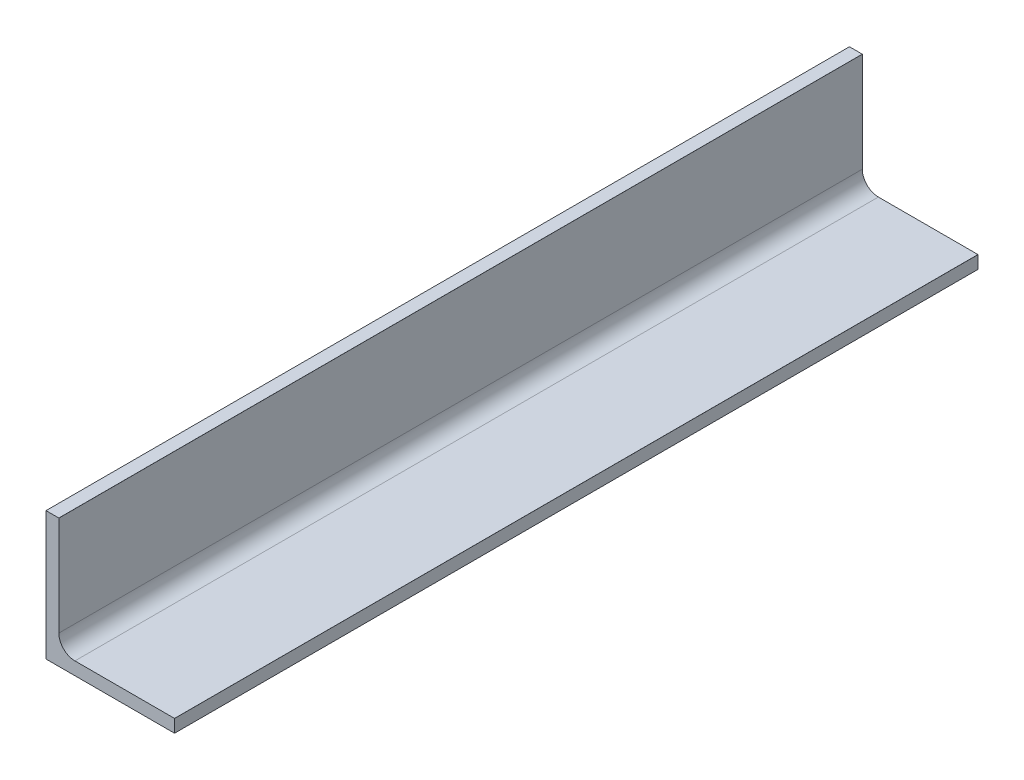
SolidWorks part; units mm, degrees
material "普通钢"
ref_plane "前视基准面" through (0, 0, 0) normal (0, 0, 1) x (1, 0, 0)
ref_plane "上视基准面" through (0, 0, 0) normal (0, 1, 0) x (1, 0, 0)
ref_plane "右视基准面" through (0, 0, 0) normal (1, 0, 0) x (0, 0, -1)
sketch "草图1" plane through (0, 0, 0) normal (0, 0, 1) x (1, 0, 0)
  line L0 (0, 0) -> (0, 40)
  line L1 (0, 40) -> (3.99, 40)
  line L2 (4, 39.99) -> (4, 9)
  line L3 (9, 4) -> (39.99, 4)
  line L4 (40, 3.99) -> (40, 0)
  line L5 (40, 0) -> (0, 0)
  arc A0 (4, 39.99) -> (3.99, 40) centre (3.99, 39.99) ccw
  arc A1 (9, 4) -> (4, 9) centre (9, 9) cw
  arc A2 (40, 3.99) -> (39.99, 4) centre (39.99, 3.99) ccw
  point P9 (4, 40)
  point P14 (40, 4)
extrude "拉伸1" add sketch "草图1" along normal blind 250
equation "\"D2@草图1\" = \"D1@草图1\""
equation "\"D4@草图1\" = \"D3@草图1\""
equation "\"D7@草图1\" = \"D5@草图1\""
